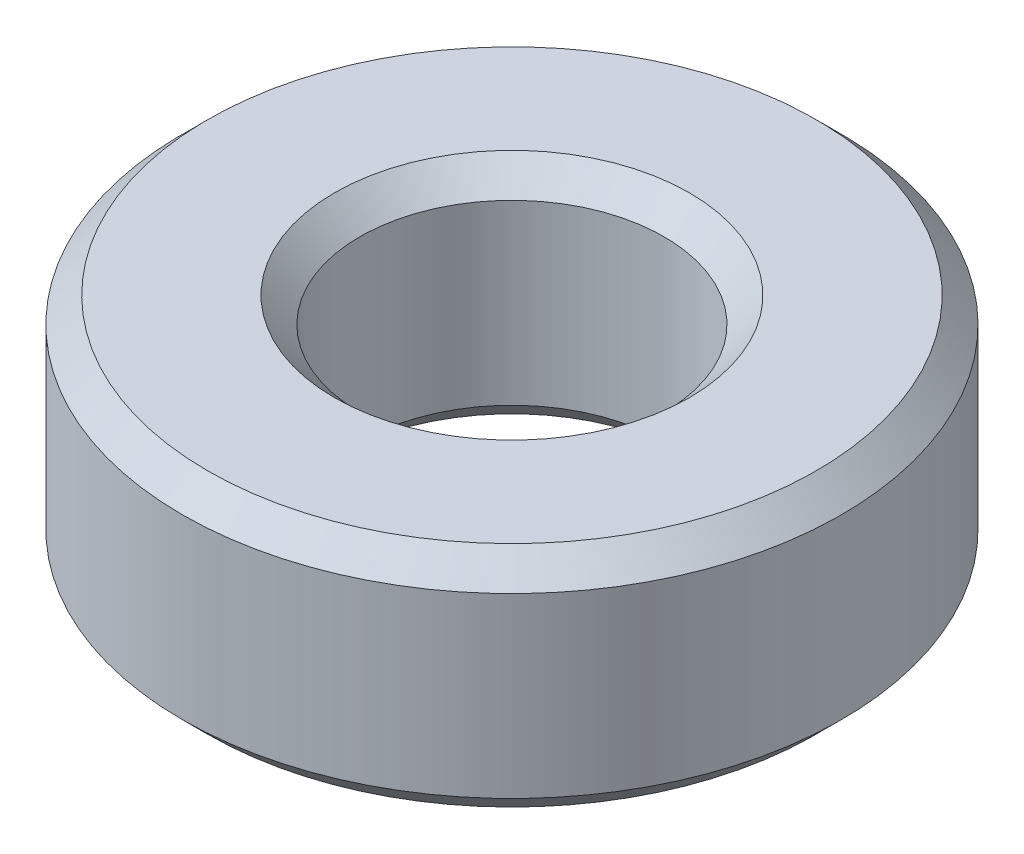
SolidWorks part; units mm, degrees
material "20#"
ref_plane "Front Plane" through (0, 0, 0) normal (0, 0, 1) x (1, 0, 0)
ref_plane "Top Plane" through (0, 0, 0) normal (0, 1, 0) x (1, 0, 0)
ref_plane "Right Plane" through (0, 0, 0) normal (1, 0, 0) x (0, 0, -1)
sketch "Sketch1" plane through (0, 0, 0) normal (0, 1, 0) x (1, 0, 0)
  circle A0 centre (0, 0) radius 3
  circle A1 centre (0, 0) radius 6.5
  dimension "D1" = 13
  dimension "D2" = 6
extrude "Boss-Extrude1" add sketch "Sketch1" along normal blind 4.5
chamfer "Chamfer1" distance 0.5 angle 45 4 edges at (0, 0, 3) (0, 4.5, 3) (0, 0, 6.5) (0, 4.5, 6.5)
